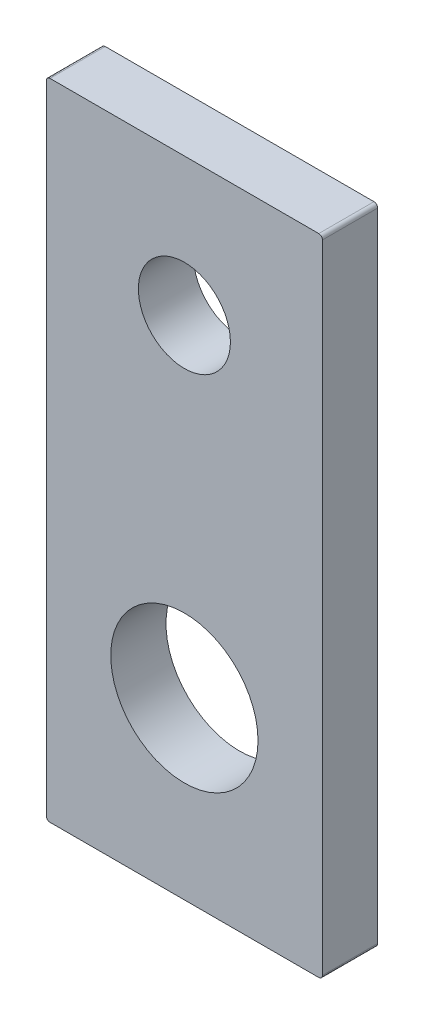
SolidWorks part; units mm, degrees
ref_plane "Front Plane" through (0, 0, 0) normal (0, 0, 1) x (1, 0, 0)
ref_plane "Top Plane" through (0, 0, 0) normal (0, 1, 0) x (1, 0, 0)
ref_plane "Right Plane" through (0, 0, 0) normal (1, 0, 0) x (0, 0, -1)
sketch "Sketch1" plane through (0, 0, 0) normal (0, 0, 1) x (1, 0, 0)
  line L1 (75, 175) -> (-75, 175)
  line L2 (75, 175) -> (75, -175)
  line L3 (75, -175) -> (-75, -175)
  line L4 (-75, 175) -> (-75, -175)
  line L5 (75, 175) -> (-75, -175) construction
  line L6 (75, -175) -> (-75, 175) construction
  point P0 (0, 0)
  dimension "D1" = 150
  dimension "D2" = 350
extrude "Boss-Extrude1" add sketch "Sketch1" along normal blind 30
sketch "Sketch2" plane through (0, 0, 30) normal (0, 0, 1) x (1, 0, 0)
  line L0 (0, 0) -> (0, 100)
  line L1 (75, 175) -> (-75, 175) construction
  line L2 (0, 0) -> (0, -80)
  line L3 (-75, -175) -> (75, -175) construction
  circle A1 centre (0, 100) radius 25
  circle A2 centre (0, -80) radius 40
  dimension "D3" = 50
  dimension "D4" = 80
  dimension "D1" = 75
  dimension "D2" = 95
extrude "Cut-Extrude1" cut sketch "Sketch2" against normal blind 30
fillet "Fillet1" radius 2 4 edges at (75, 175, 15) (75, -175, 15) (-75, -175, 15) (-75, 175, 15)
